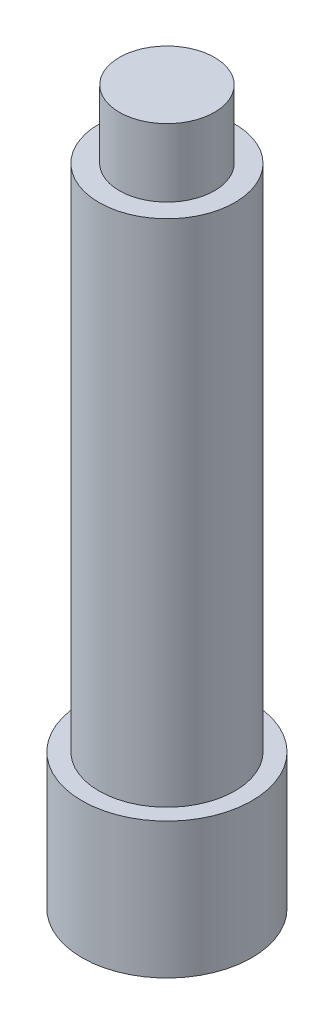
SolidWorks part; units mm, degrees
ref_plane "Front Plane" through (0, 0, 0) normal (0, 0, 1) x (1, 0, 0)
ref_plane "Top Plane" through (0, 0, 0) normal (0, 1, 0) x (1, 0, 0)
ref_plane "Right Plane" through (0, 0, 0) normal (1, 0, 0) x (0, 0, -1)
other "Configuration Table"
sketch "Sketch1" plane through (0, 0, 0) normal (0, 1, 0) x (1, 0, 0)
  circle A0 centre (0, 0) radius 12.5
  dimension "D1" = 25
extrude "Boss-Extrude1" add sketch "Sketch1" along normal blind 20
sketch "Sketch2" plane through (0, 20, 0) normal (0, 1, 0) x (1, 0, 0)
  circle A0 centre (0, 0) radius 10
  dimension "D1" = 20
extrude "Boss-Extrude2" add sketch "Sketch2" along normal blind 75 contours A0
sketch "Sketch3" plane through (0, 95, 0) normal (0, 1, 0) x (1, 0, 0)
  circle A0 centre (0, 0) radius 7
  dimension "D1" = 14
extrude "Boss-Extrude3" add sketch "Sketch3" along normal blind 10
